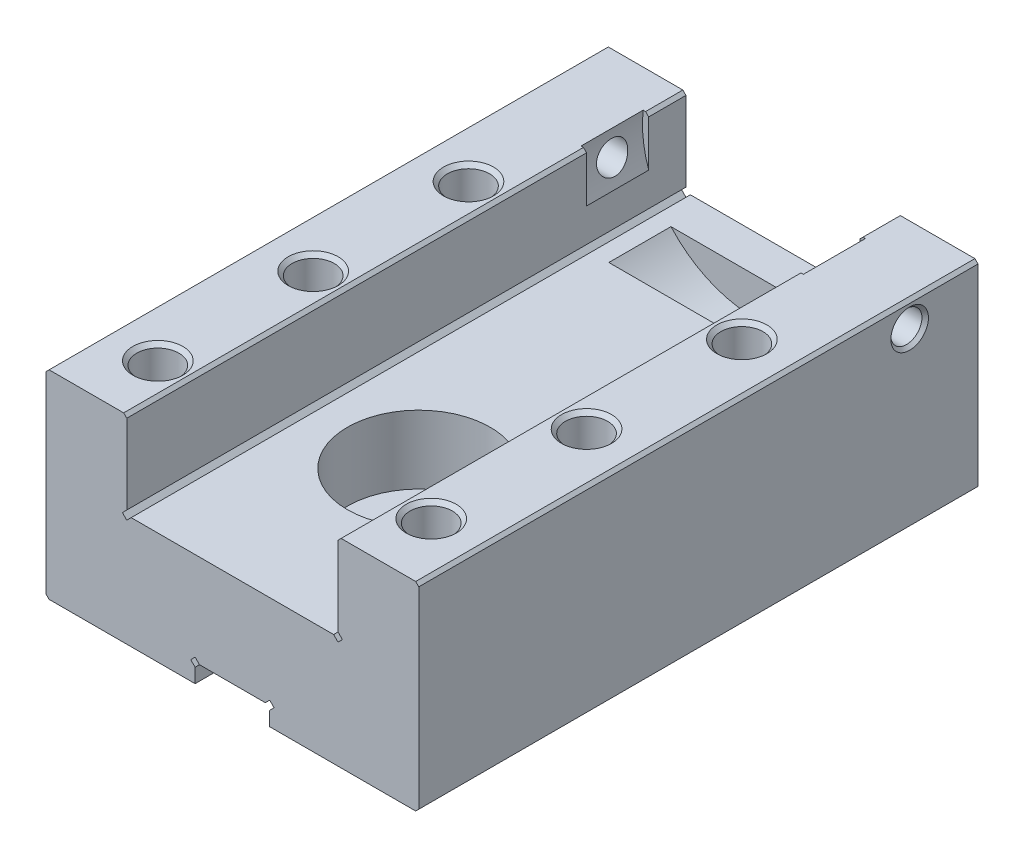
from build123d import *

# Parameters (mm, degrees)
BOSS_EXTRUDE1_DEPTH                   = 90
SKETCH2_R                             = 11.5
CUT_EXTRUDE1_DEPTH                    = 11
SKETCH3_R                             = 6
CUT_EXTRUDE2_DEPTH                    = 99.107084352
CUT_EXTRUDE3_START                    = -6
SKETCH4_R                             = 18
CUT_EXTRUDE3_DEPTH                    = 10
M8_TAPPED_HOLE1_D                     = 6.8
M8_TAPPED_HOLE1_DEPTH                 = 16
M8_TAPPED_HOLE1_CSINK_D               = 8.05
M8_TAPPED_HOLE1_CSINK_ANGLE           = 90
M8_TAPPED_HOLE1_TIP                   = 2.042926105
M6_TAPPED_HOLE1_D                     = 5
M6_TAPPED_HOLE1_CSINK_D               = 6.05
M6_TAPPED_HOLE1_CSINK_ANGLE           = 90
M5_TAPPED_HOLE1_D                     = 4.2
M5_TAPPED_HOLE1_CSINK_D               = 5.05
M5_TAPPED_HOLE1_CSINK_ANGLE           = 90
M5_TAPPED_HOLE2_D                     = 4.2
M5_TAPPED_HOLE2_DEPTH                 = 11
M5_TAPPED_HOLE2_CSINK_D               = 5.05
M5_TAPPED_HOLE2_CSINK_ANGLE           = 90
M5_TAPPED_HOLE2_TIP                   = 1.2618073
M5_TAPPED_HOLE2_ON_FACE_2_D           = 4.2
M5_TAPPED_HOLE2_ON_FACE_2_DEPTH       = 11
M5_TAPPED_HOLE2_ON_FACE_2_CSINK_D     = 5.05
M5_TAPPED_HOLE2_ON_FACE_2_CSINK_ANGLE = 90
M5_TAPPED_HOLE2_ON_FACE_2_TIP         = 1.2618073


with BuildPart() as part:
    # Sketch1 → Boss-Extrude1 (new body)
    with BuildSketch(Plane.XY):
        Polygon((-6, 0), (-29.5, 0), (-30, 0.5), (-30, 31.5), (-29.5, 32), (-17.5, 32), (-17, 31.5), (-17, 18.707106781), (-17.707106781, 18), (-17, 17.292893219), (-16.292893219, 18), (16.292893219, 18), (17, 17.292893219), (17.707106781, 18), (17, 18.707106781), (17, 31.5), (17.5, 32), (29.5, 32), (30, 31.5), (30, 0.5), (29.5, 0), (6, 0), (6, 2.292893219), (6.707106781, 3), (6, 3.707106781), (5.292893219, 3), (-5.292893219, 3), (-6, 3.707106781), (-6.707106781, 3), (-6, 2.292893219), align=None)
    extrude(amount=BOSS_EXTRUDE1_DEPTH)

    # Sketch2 → Cut-Extrude1 (cut)
    with BuildSketch(Plane(origin=(0, 18, 0), x_dir=(1, 0, 0), z_dir=(0, 1, 0))):
        with Locations(Location((0, -60, 0), (0, 0, 270))):
            Circle(SKETCH2_R)
    extrude(amount=-CUT_EXTRUDE1_DEPTH, mode=Mode.SUBTRACT)

    # Sketch3 → Cut-Extrude2 (cut, through all)
    with BuildSketch(Plane(origin=(0, 7, 0), x_dir=(1, 0, 0), z_dir=(0, 1, 0))):
        with Locations(Location((0, -60, 0), (0, 0, 270))):
            Circle(SKETCH3_R)
    extrude(amount=-CUT_EXTRUDE2_DEPTH, mode=Mode.SUBTRACT)

    # Sketch4 → Cut-Extrude3 (cut)
    with BuildSketch(Plane(origin=(0, 0, 0), x_dir=(-1, 0, 0), z_dir=(0, 0, -1)).offset(CUT_EXTRUDE3_START)):
        with Locations((0, 30)):
            Circle(SKETCH4_R)
    extrude(amount=-CUT_EXTRUDE3_DEPTH, mode=Mode.SUBTRACT)

    # M8 Tapped Hole1
    with Locations(Plane(origin=(-22, 32, 30), x_dir=(0, 0, 1), z_dir=(0, 1, 0))):
        with Locations((0, 0), (25, 0), (50, 0), (0, 44), (25, 44), (50, 44)):
            CounterSinkHole(M8_TAPPED_HOLE1_D / 2, M8_TAPPED_HOLE1_CSINK_D / 2, depth=M8_TAPPED_HOLE1_DEPTH, counter_sink_angle=M8_TAPPED_HOLE1_CSINK_ANGLE)
            with Locations((0, 0, -(M8_TAPPED_HOLE1_DEPTH + M8_TAPPED_HOLE1_TIP / 2))):  # 118° drill point
                Cone(0, M8_TAPPED_HOLE1_D / 2, M8_TAPPED_HOLE1_TIP, mode=Mode.SUBTRACT)

    # M6 Tapped Hole1 (through all)
    with Locations(Plane(origin=(30, 28, 11), x_dir=(0, 1, 0), z_dir=(1, 0, 0))):
        with Locations((0, 0)):
            CounterSinkHole(M6_TAPPED_HOLE1_D / 2, M6_TAPPED_HOLE1_CSINK_D / 2, counter_sink_angle=M6_TAPPED_HOLE1_CSINK_ANGLE)

    # M5 Tapped Hole1 (through all)
    with Locations(Plane(origin=(0, 3, 11), x_dir=(0, 0, -1), z_dir=(0, -1, 0))):
        with Locations((0, 0)):
            CounterSinkHole(M5_TAPPED_HOLE1_D / 2, M5_TAPPED_HOLE1_CSINK_D / 2, counter_sink_angle=M5_TAPPED_HOLE1_CSINK_ANGLE)

    # M5 Tapped Hole2
    with Locations(Plane(origin=(0, 3, 83), x_dir=(0, 0, -1), z_dir=(0, -1, 0))):
        with Locations((0, 0)):
            CounterSinkHole(M5_TAPPED_HOLE2_D / 2, M5_TAPPED_HOLE2_CSINK_D / 2, depth=M5_TAPPED_HOLE2_DEPTH, counter_sink_angle=M5_TAPPED_HOLE2_CSINK_ANGLE)
            with Locations((0, 0, -(M5_TAPPED_HOLE2_DEPTH + M5_TAPPED_HOLE2_TIP / 2))):  # 118° drill point
                Cone(0, M5_TAPPED_HOLE2_D / 2, M5_TAPPED_HOLE2_TIP, mode=Mode.SUBTRACT)

    # M5 Tapped Hole2 on face 2
    with Locations(Plane(origin=(23, 0, 60), x_dir=(0, 0, -1), z_dir=(0, -1, 0))):
        with Locations((0, 0), (0, -46)):
            CounterSinkHole(M5_TAPPED_HOLE2_ON_FACE_2_D / 2, M5_TAPPED_HOLE2_ON_FACE_2_CSINK_D / 2, depth=M5_TAPPED_HOLE2_ON_FACE_2_DEPTH, counter_sink_angle=M5_TAPPED_HOLE2_ON_FACE_2_CSINK_ANGLE)
            with Locations((0, 0, -(M5_TAPPED_HOLE2_ON_FACE_2_DEPTH + M5_TAPPED_HOLE2_ON_FACE_2_TIP / 2))):  # 118° drill point
                Cone(0, M5_TAPPED_HOLE2_ON_FACE_2_D / 2, M5_TAPPED_HOLE2_ON_FACE_2_TIP, mode=Mode.SUBTRACT)


solid = part.part
